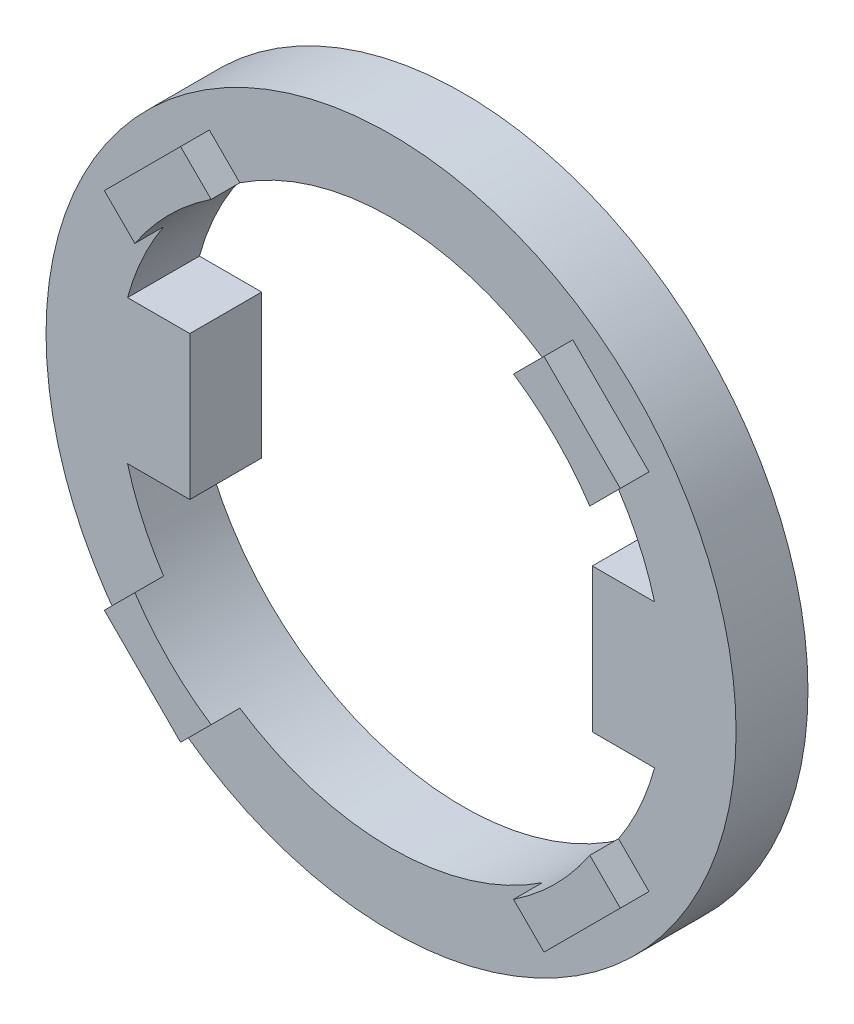
from build123d import *

# Parameters (mm, degrees)
SKETCH_1_R      = 24
EXTRUDE_1_DEPTH = 5
EXTRUDE_2_DEPTH = 2


with BuildPart() as part:
    # 草图1 → 凸台-拉伸1 (new body)
    with BuildSketch(Plane.XY):
        Circle(SKETCH_1_R)
        with BuildLine():
            Line((-18.33030278, 5), (-14, 5))
            Line((-14, 5), (-14, -5))
            Line((-14, -5), (-18.33030278, -5))
            ThreePointArc((-18.33030278, -5), (0, -19), (18.33030278, -5))
            Line((18.33030278, -5), (14, -5))
            Line((14, -5), (14, 5))
            Line((14, 5), (18.33030278, 5))
            ThreePointArc((18.33030278, 5), (0, 19), (-18.33030278, 5))
        make_face(mode=Mode.SUBTRACT)
    extrude(amount=EXTRUDE_1_DEPTH)

    # 草图2 → 凸台-拉伸2 (add)
    with BuildSketch(Plane.XY.offset(5)):
        with BuildLine():
            Line((-15.822404015, 10.519103156), (-17.943724358, 12.640423499))
            Line((-17.943724358, 12.640423499), (-12.640423499, 17.943724358))
            Line((-12.640423499, 17.943724358), (-10.519103156, 15.822404015))
            ThreePointArc((-10.519103156, 15.822404015), (-13.435028843, 13.435028843), (-15.822404015, 10.519103156))
        make_face()
        with BuildLine():
            Line((10.519103156, 15.822404015), (12.640423499, 17.943724358))
            Line((12.640423499, 17.943724358), (17.943724358, 12.640423499))
            Line((17.943724358, 12.640423499), (15.822404015, 10.519103156))
            ThreePointArc((15.822404015, 10.519103156), (13.435028843, 13.435028843), (10.519103156, 15.822404015))
        make_face()
        with BuildLine():
            Line((15.822404015, -10.519103156), (17.943724358, -12.640423499))
            Line((17.943724358, -12.640423499), (12.640423499, -17.943724358))
            Line((12.640423499, -17.943724358), (10.519103156, -15.822404015))
            ThreePointArc((10.519103156, -15.822404015), (13.435028843, -13.435028843), (15.822404015, -10.519103156))
        make_face()
        with BuildLine():
            Line((-10.519103156, -15.822404015), (-12.640423499, -17.943724358))
            Line((-12.640423499, -17.943724358), (-17.943724358, -12.640423499))
            Line((-17.943724358, -12.640423499), (-15.822404015, -10.519103156))
            ThreePointArc((-15.822404015, -10.519103156), (-13.435028843, -13.435028843), (-10.519103156, -15.822404015))
        make_face()
    extrude(amount=EXTRUDE_2_DEPTH)


solid = part.part
